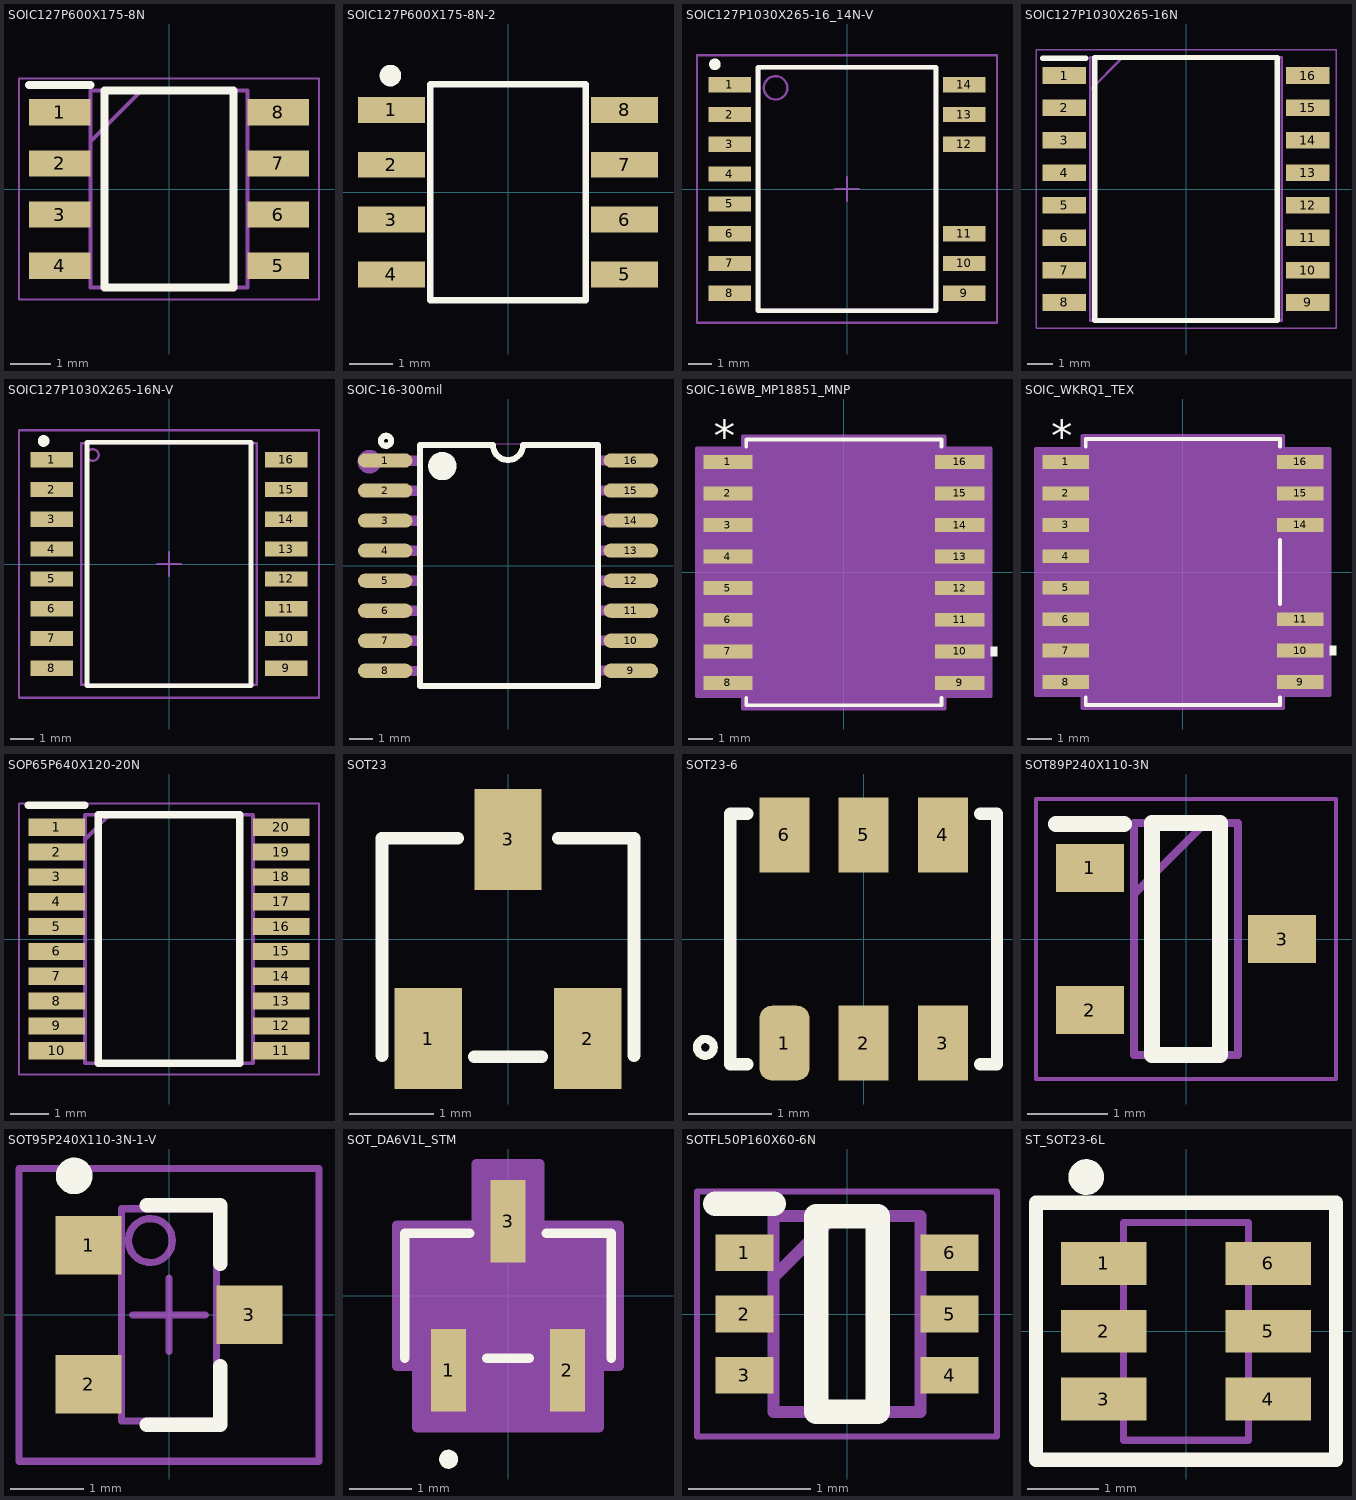
[diagram p0: the footprints below, top view; thin cyan lines are the x and y axes]
# Altium footprint library MISC82254-2.PcbLib: 93 footprints (part 5 of 6)
Each footprint in its own frame and in the unit in brackets; x right, y up, seen from the top. Pads: shape width x height; smd on the part's side, far side on the other; paste and mask are expansions set on the pad; w line width, h text height; cw(c..) or ccw(c..) is an arc to the next point about the centre after c.

## SOIC127P600X175-8N [mm]
pads (8):
  rect 1.525x0.65 smd: 1(-2.712,1.905) 2(-2.712,0.635) 3(-2.712,-0.635) 4(-2.712,-1.905) 5(2.712,-1.905) 6(2.712,-0.635) 7(2.712,0.635) 8(2.712,1.905)
Top Overlay:
  lines w0.2: -3.475,2.58 -1.95,2.58 ; -1.6,-2.45 1.6,-2.45 1.6,2.45 -1.6,2.45 -1.6,-2.45
Mechanical 13:
  lines w0.1: -1.95,1.18 -0.68,2.45 ; -1.95,-2.45 1.95,-2.45 1.95,2.45 -1.95,2.45 -1.95,-2.45
Mechanical 15:
  lines w0.05: -3.725,-2.75 3.725,-2.75 3.725,2.75 -3.725,2.75 -3.725,-2.75
3D body "NE555DR.stp": height 1.75, standoff 0, extent -3,-2.45 3,2.45

## SOIC127P600X175-8N-2 [mm] "SOIC,1.27mm pitch;8 pin,3.90mm W X 4.90mm L X 1.75mm H body"
height 1.75
pads (8):
  rect 1.55x0.6 smd paste+0 mask+0: 1(-2.7,1.905) 2(-2.7,0.635) 3(-2.7,-0.635) 4(-2.7,-1.905) 5(2.7,-1.905) 6(2.7,-0.635) 7(2.7,0.635) 8(2.7,1.905)
Top Overlay:
  circle w0.25: c-2.725,2.7 r0.125
  lines w0.15: -1.8,-2.5 -1.8,2.5 1.8,2.5 1.8,-2.5 -1.8,-2.5
3D body "DSO-8-1.stp": height 1.76, standoff 0, extent -3,-2.5 3,2.5

## SOIC127P1030X265-16_14N-V [mm] "SOIC,1.27mm,pitch;14 pin,7.50mm W X 10.30mm L X 2.65mm H body"
height 2.65
pads (14):
  rect 1.8x0.65 smd paste+0 mask+0: 1(-5,4.445) 2(-5,3.175) 3(-5,1.905) 4(-5,0.635) 5(-5,-0.635) 6(-5,-1.905) 7(-5,-3.175) 8(-5,-4.445) 9(5,-4.445) 10(5,-3.175) 11(5,-1.905) 12(5,1.905) 13(5,3.175) 14(5,4.445)
Top Overlay:
  circle w0.25: c-5.638,5.32 r0.125
  lines w0.2: -3.8,-5.2 -3.8,5.2 3.8,5.2 3.8,-5.2 -3.8,-5.2
Mechanical 3:
  text ".DESIGNATOR" at 0,0 h1.2
Mechanical 13:
  circle w0.1: c-3.048,4.318 r0.5
  lines w0.1: -3.75,-5.15 -3.75,5.15 3.75,5.15 3.75,-5.15 -3.75,-5.15
Mechanical 15:
  lines w0.1: -0.5,0 0.5,0 ; 0,-0.5 0,0.5 ; -6.4,-5.7 -6.4,5.7 6.4,5.7 6.4,-5.7 -6.4,-5.7
3D body "PG-DSO-14.STEP": height 2.65, standoff 0, extent -5.15,-5.15 5.15,5.15

## SOIC127P1030X265-16N [mm]
pads (16):
  rect 1.7x0.65 smd: 1(-4.775,4.445) 2(-4.775,3.175) 3(-4.775,1.905) 4(-4.775,0.635) 5(-4.775,-0.635) 6(-4.775,-1.905) 7(-4.775,-3.175) 8(-4.775,-4.445) 9(4.775,-4.445) 10(4.775,-3.175) 11(4.775,-1.905) 12(4.775,-0.635) 13(4.775,0.635) 14(4.775,1.905) 15(4.775,3.175) 16(4.775,4.445)
Top Overlay:
  lines w0.2: -5.625,5.12 -3.925,5.12 ; -3.575,-5.15 -3.575,5.15 3.575,5.15 3.575,-5.15 -3.575,-5.15
Mechanical 13:
  lines w0.1: -3.75,3.88 -2.48,5.15 ; -3.75,-5.15 -3.75,5.15 3.75,5.15 3.75,-5.15 -3.75,-5.15
Mechanical 15:
  lines w0.05: -5.875,-5.45 -5.875,5.45 5.875,5.45 5.875,-5.45 -5.875,-5.45
3D body "NSI6602B-DSWR.stp": height 2.65, standoff 0, extent -5.15,-5.15 5.15,5.15

## SOIC127P1030X265-16N-V [mm] "SOIC,1.27mm pitch;16 pin,7.50mm W X 10.30mm L X 2.65mm H body"
height 2.65
pads (16):
  rect 1.8x0.65 smd paste+0 mask+0: 1(-5,4.445) 2(-5,3.175) 3(-5,1.905) 4(-5,0.635) 5(-5,-0.635) 6(-5,-1.905) 7(-5,-3.175) 8(-5,-4.445) 9(5,-4.445) 10(5,-3.175) 11(5,-1.905) 12(5,-0.635) 13(5,0.635) 14(5,1.905) 15(5,3.175) 16(5,4.445)
Top Overlay:
  circle w0.25: c-5.35,5.25 r0.125
  lines w0.2: -3.5,-5.2 3.5,-5.2 3.5,5.2 -3.5,5.2 -3.5,-5.2
Mechanical 3:
  text ".DESIGNATOR" at 0,0 h1.2
Mechanical 13:
  circle w0.1: c-3.25,4.65 r0.25
  lines w0.1: -3.75,-5.15 3.75,-5.15 3.75,5.15 -3.75,5.15 -3.75,-5.15
Mechanical 15:
  lines w0.1: -0.5,0 0.5,0 ; 0,-0.5 0,0.5 ; -6.4,-5.7 6.4,-5.7 6.4,5.7 -6.4,5.7 -6.4,-5.7
3D body "DSO-16-30.stp": height 2.66, standoff 0, extent -5.15,-5.15 5.15,5.15

## SOIC-16-300mil [mm]
pads (16):
  oval 2.3x0.6 smd paste+0 mask+0.05: 1(-5.194,4.445) 2(-5.194,3.175) 3(-5.194,1.905) 4(-5.194,0.635) 5(-5.194,-0.635) 6(-5.194,-1.905) 7(-5.194,-3.175) 8(-5.194,-4.445) 9(5.194,-4.445) 10(5.194,-3.175) 11(5.194,-1.905) 12(5.194,-0.635) 13(5.194,0.635) 14(5.194,1.905) 15(5.194,3.175) 16(5.194,4.445)
Top Overlay:
  circle w0.254: c-5.16,5.28 r0.215
  lines w0.254: -3.721,-5.1 -3.721,5.1 -0.635,5.1 ccw(c0,5.1) 0.635,5.1 3.797,5.1 3.797,-5.1 -3.721,-5.1
  lines w0.6: -2.477,4.211 cw(c-2.777,4.214) -2.477,4.216
Mechanical 6:
  circle w0.5: c-5.86,4.4 r0.25
Mechanical 15:
  drawing of 37 lines, arcs and shapes, not listed
3D body "NSI6602B-DSWR.stp": height 2.65, standoff 0, extent -5.15,-5.15 5.15,5.15

## SOIC-16WB_MP18851_MNP [mil]
pads (16):
  rect 78x22 smd paste+0 mask+0: 1(-183.5,175) 2(-183.5,125) 3(-183.5,75) 4(-183.5,25) 5(-183.5,-25) 6(-183.5,-75) 7(-183.5,-125) 8(-183.5,-175) 9(183.5,-175) 10(183.5,-125) 11(183.5,-75) 12(183.5,-25) 13(183.5,25) 14(183.5,75) 15(183.5,125) 16(183.5,175)
Top Overlay:
  region: 232.5,-117.5 242.5,-117.5 242.5,-132.5 232.5,-132.5
  lines w6: -154.5,-199.1 -154.5,-210.5 154.5,-210.5 154.5,-199.1 ; -154.5,199.1 -154.5,210.5 154.5,210.5 154.5,199.1
  text "*" at -206,192 h50
Mechanical 13:
  lines w0: -12,205.5 ccw(c0,205.5) 12,205.5
  lines w1: -208.5,-185 -208.5,-165 -149.5,-165 -149.5,-185 -208.5,-185 ; -208.5,-135 -208.5,-115 -149.5,-115 -149.5,-135 -208.5,-135 ; -208.5,-85 -208.5,-65 -149.5,-65 -149.5,-85 -208.5,-85 ; -208.5,-35 -208.5,-15 -149.5,-15 -149.5,-35 -208.5,-35 ; -208.5,15 -208.5,35 -149.5,35 -149.5,15 -208.5,15 ; -208.5,65 -208.5,85 -149.5,85 -149.5,65 -208.5,65 ; -208.5,115 -208.5,135 -149.5,135 -149.5,115 -208.5,115 ; -208.5,165 -208.5,185 -149.5,185 -149.5,165 -208.5,165 ; -149.5,-205.5 149.5,-205.5 149.5,205.5 -149.5,205.5 -149.5,-205.5 ; 149.5,-185 149.5,-165 208.5,-165 208.5,-185 149.5,-185 ; 149.5,-135 149.5,-115 208.5,-115 208.5,-135 149.5,-135 ; 149.5,-85 149.5,-65 208.5,-65 208.5,-85 149.5,-85 ; 149.5,-35 149.5,-15 208.5,-15 208.5,-35 149.5,-35 ; 149.5,15 149.5,35 208.5,35 208.5,15 149.5,15 ; 149.5,65 149.5,85 208.5,85 208.5,65 149.5,65 ; 149.5,115 149.5,135 208.5,135 208.5,115 149.5,115 ; 149.5,165 149.5,185 208.5,185 208.5,165 149.5,165
  text "*" at -147,152.5 h50
Mechanical 15:
  region: -159.5,-196 -232.5,-196 -232.5,196 -159.5,196 -159.5,215.5 159.5,215.5 159.5,196 232.5,196 232.5,-196 159.5,-196 159.5,-215.5 -159.5,-215.5
  lines w6: -232.5,-196 -232.5,196 -159.5,196 -159.5,215.5 159.5,215.5 159.5,196 232.5,196 232.5,-196 159.5,-196 159.5,-215.5 -159.5,-215.5 -159.5,-196 -232.5,-196
3D body "SOIC-16WB_MP18851_MNP.step": height 104.09, standoff 0, extent -208.5,-205.51 208.5,205.51

## SOIC_WKRQ1_TEX [mil]
pads (14):
  rect 74x22 smd paste+0 mask+0: 1(-186.5,175) 2(-186.5,125) 3(-186.5,75) 4(-186.5,25) 5(-186.5,-25) 6(-186.5,-75) 7(-186.5,-125) 8(-186.5,-175) 9(186.5,-175) 10(186.5,-125) 11(186.5,-75) 14(186.5,75) 15(186.5,125) 16(186.5,175)
Top Overlay:
  region: 233.5,-117.5 243.5,-117.5 243.5,-132.5 233.5,-132.5
  lines w6: -154.5,-199.1 -154.5,-211.5 154.5,-211.5 154.5,-199.1 ; -154.5,199.1 -154.5,211.5 154.5,211.5 154.5,199.1 ; 154.5,-50.9 154.5,50.9
  text "*" at -209,192 h50
Mechanical 13:
  lines w0: -12,206.5 ccw(c0,206.5) 12,206.5
  lines w1: -209.5,-185 -209.5,-165 -149.5,-165 -149.5,-185 -209.5,-185 ; -209.5,-135 -209.5,-115 -149.5,-115 -149.5,-135 -209.5,-135 ; -209.5,-85 -209.5,-65 -149.5,-65 -149.5,-85 -209.5,-85 ; -209.5,-35 -209.5,-15 -149.5,-15 -149.5,-35 -209.5,-35 ; -209.5,15 -209.5,35 -149.5,35 -149.5,15 -209.5,15 ; -209.5,65 -209.5,85 -149.5,85 -149.5,65 -209.5,65 ; -209.5,115 -209.5,135 -149.5,135 -149.5,115 -209.5,115 ; -209.5,165 -209.5,185 -149.5,185 -149.5,165 -209.5,165 ; -149.5,-206.5 149.5,-206.5 149.5,206.5 -149.5,206.5 -149.5,-206.5 ; 149.5,-185 149.5,-165 209.5,-165 209.5,-185 149.5,-185 ; 149.5,-135 149.5,-115 209.5,-115 209.5,-135 149.5,-135 ; 149.5,-85 149.5,-65 209.5,-65 209.5,-85 149.5,-85 ; 149.5,65 149.5,85 209.5,85 209.5,65 149.5,65 ; 149.5,115 149.5,135 209.5,135 209.5,115 149.5,115 ; 149.5,165 149.5,185 209.5,185 209.5,165 149.5,165
  text "*" at -147,153.5 h50
Mechanical 15:
  region: -159.5,-196 -233.5,-196 -233.5,196 -159.5,196 -159.5,216.5 159.5,216.5 159.5,196 233.5,196 233.5,-196 159.5,-196 159.5,-216.5 -159.5,-216.5
  lines w6: -233.5,-196 -233.5,196 -159.5,196 -159.5,216.5 159.5,216.5 159.5,196 233.5,196 233.5,-196 159.5,-196 159.5,-216.5 -159.5,-216.5 -159.5,-196 -233.5,-196
3D body "SOIC_WKRQ1_TEX.step": height 104.09, standoff 0, extent -209.49,-206.5 209.49,206.5

## SOP65P640X120-20N [mm]
pads (20):
  rect 1.475x0.45 smd: 1(-2.938,2.925) 2(-2.938,2.275) 3(-2.938,1.625) 4(-2.938,0.975) 5(-2.938,0.325) 6(-2.938,-0.325) 7(-2.938,-0.975) 8(-2.938,-1.625) 9(-2.938,-2.275) 10(-2.938,-2.925) 11(2.938,-2.925) 12(2.938,-2.275) 13(2.938,-1.625) 14(2.938,-0.975) 15(2.938,-0.325) 16(2.938,0.325) 17(2.938,0.975) 18(2.938,1.625) 19(2.938,2.275) 20(2.938,2.925)
Top Overlay:
  lines w0.2: -3.675,3.5 -2.2,3.5 ; -1.85,-3.25 -1.85,3.25 1.85,3.25 1.85,-3.25 -1.85,-3.25
Mechanical 13:
  lines w0.1: -2.2,2.6 -1.55,3.25 ; -2.2,-3.25 -2.2,3.25 2.2,3.25 2.2,-3.25 -2.2,-3.25
Mechanical 15:
  lines w0.05: -3.925,-3.55 -3.925,3.55 3.925,3.55 3.925,-3.55 -3.925,-3.55
3D body "SN74ACT244PWR.stp": height 1.13, standoff 0, extent -3.2,-3.25 3.2,3.25

## SOT23 [mm]
height 2.55
pads (3):
  rect 0.8x1.2 smd: 1(-0.95,-1.185) 2(0.95,-1.185) 3(0,1.185)
Top Overlay:
  lines w0.15: -1.5,-1.386 -1.5,1.2 -0.6,1.2 ; -0.4,-1.4 0.4,-1.4 ; 0.6,1.2 1.5,1.2 1.5,-1.386
3D body "SOT23.step": height 0.95, standoff 0, extent -1.45,-1.177 1.45,1.123

## SOT23-6 [mm]
height 1.45
pads (6):
  rrect50% 0.6x0.9 smd: 1(-0.95,-1.25)
  rect 0.6x0.9 smd: 2(0,-1.25) 3(0.95,-1.25) 4(0.95,1.25) 5(0,1.25) 6(-0.95,1.25)
Top Overlay:
  circle w0.1: c-1.9,-1.3 r0.1
  lines w0.15: -1.4,-1.5 -1.6,-1.5 -1.6,1.5 -1.4,1.5 ; 1.4,-1.5 1.6,-1.5 1.6,1.5 1.4,1.5
3D body "SOT23-6.step": height 1.2, standoff 0, extent -1.448,-1.249 1.452,1.351

## SOT89P240X110-3N [mm]
pads (3):
  rect 0.85x0.6 smd: 1(-1.2,0.89) 2(-1.2,-0.89) 3(1.2,0)
Top Overlay:
  lines w0.2: -1.625,1.44 -0.775,1.44 ; -0.425,-1.45 0.425,-1.45 0.425,1.45 -0.425,1.45 -0.425,-1.45
Mechanical 13:
  lines w0.1: -0.65,0.56 0.24,1.45 ; -0.65,-1.45 0.65,-1.45 0.65,1.45 -0.65,1.45 -0.65,-1.45
Mechanical 15:
  lines w0.05: -1.875,-1.75 1.875,-1.75 1.875,1.75 -1.875,1.75 -1.875,-1.75
3D body "AZ431LANTR-G1.stp": height 1.1, standoff 0, extent -1.2,-1.45 1.2,1.45

## SOT95P240X110-3N-1-V [mm] "SOT,0.95mm pitch;3 pin,1.30mm W X 2.90mm L X 1.10mm H body"
height 1.1
pads (3):
  rect 0.9x0.8 smd paste+0 mask+0: 1(-1.1,0.95) 2(-1.1,-0.95) 3(1.1,0)
Top Overlay:
  circle w0.25: c-1.295,1.9 r0.125
  lines w0.2: -0.3,-1.5 0.7,-1.5 0.7,-0.7 ; -0.3,1.5 0.7,1.5 0.7,0.7
Mechanical 3:
  text ".DESIGNATOR" at -3.643,-0.385 h1.2
Mechanical 13:
  circle w0.1: c-0.254,1.016 r0.3
  lines w0.1: -0.65,-1.45 0.65,-1.45 0.65,1.45 -0.65,1.45 -0.65,-1.45
Mechanical 15:
  lines w0.1: -0.5,0 0.5,0 ; 0,-0.5 0,0.5 ; -2.05,-2 2.05,-2 2.05,2 -2.05,2 -2.05,-2
3D body "SOT-23-3-11.stp": height 1.1, standoff 0, extent -1.2,-1.45 1.2,1.45

## SOT_DA6V1L_STM [mil]
pads (3):
  rect 22x52 smd paste+0 mask+0: 1(-37.4,-47) 2(37.4,-47) 3(0,47)
Top Overlay:
  circle w6: c-37.4,-103 r3
  lines w6: -65,-39.5 -65,39.5 -24.1,39.5 ; -13.3,-39.5 13.3,-39.5 ; 24.1,39.5 65,39.5 65,-39.5
Mechanical 13:
  circle w0: c-37.4,-24.5 r3
  lines w1: -60,-34.5 60,-34.5 60,34.5 -60,34.5 -60,-34.5 ; -47.4,-59 -47.4,-34.5 -27.4,-34.5 -27.4,-59 -47.4,-59 ; -10,34.5 10,34.5 10,59 -10,59 -10,34.5 ; 27.4,-59 27.4,-34.5 47.4,-34.5 47.4,-59 27.4,-59
Mechanical 15:
  region: -70,-44.5 -70,44.5 -20,44.5 -20,83 20,83 20,44.5 70,44.5 70,-44.5 57.4,-44.5 57.4,-83 -57.4,-83 -57.4,-44.5
  lines w6: -70,-44.5 -70,44.5 -20,44.5 -20,83 20,83 20,44.5 70,44.5 70,-44.5 57.4,-44.5 57.4,-83 -57.4,-83 -57.4,-44.5 -70,-44.5
3D body "SOT_DA6V1L_STM.step": height 55.12, standoff 0, extent -60,-59.02 60,59.02

## SOTFL50P160X60-6N [mm]
pads (6):
  rect 0.475x0.3 smd: 1(-0.838,0.5) 2(-0.838,0) 3(-0.838,-0.5) 4(0.838,-0.5) 5(0.838,0) 6(0.838,0.5)
Top Overlay:
  lines w0.2: -1.075,0.9 -0.6,0.9 ; -0.25,-0.8 0.25,-0.8 0.25,0.8 -0.25,0.8 -0.25,-0.8
Mechanical 13:
  lines w0.1: -0.6,0.3 -0.1,0.8 ; -0.6,-0.8 0.6,-0.8 0.6,0.8 -0.6,0.8 -0.6,-0.8
Mechanical 15:
  lines w0.05: -1.225,-1 1.225,-1 1.225,1 -1.225,1 -1.225,-1
3D body "TPS562242DRLR.stp": height 0.6, standoff 0, extent -0.8,-0.78 0.8,0.82

## ST_SOT23-6L [mm] "SOT23, 6-Leads, Body 2.93x2.80mm, Pitch 0.95mm, IPC Medium Density"
height 1.45
pads (6):
  rect 1.2x0.6 smd: 1(-1.15,0.95) 2(-1.15,0) 3(-1.15,-0.95) 4(1.15,-0.95) 5(1.15,0) 6(1.15,0.95)
Top Overlay:
  circle w0.25: c-1.397,2.159 r0.125
  lines w0.2: -2.1,-1.8 -2.1,1.8 2.1,1.8 2.1,-1.8 -2.1,-1.8
Mechanical 13:
  lines w0.1: -0.875,-1.525 0.875,-1.525 0.875,1.525 -0.875,1.525 -0.875,-1.525
3D body "ST_SOT23-6L.step": height 1.45, standoff 0, extent -1.6,-1.525 1.6,1.525